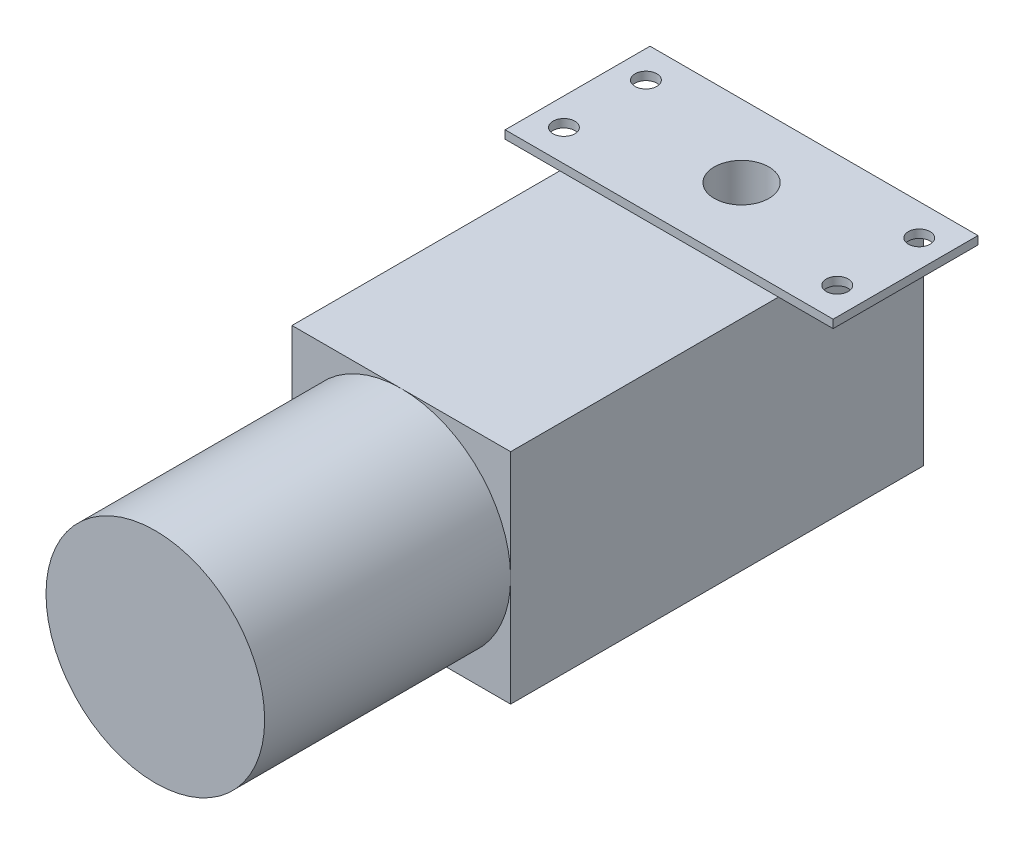
from build123d import *

# Parameters (mm, degrees)
SKETCH_1_W          = 80
SKETCH_1_H          = 80
EXTRUDE_1_DEPTH     = 241
SKETCH_2_W          = 120
SKETCH_2_H          = 53
EXTRUDE_2_DEPTH     = 3
SKETCH_3_R          = 4
CUT_EXTRUDE_1_DEPTH = 262.858740545
SKETCH_4_R          = 10
CUT_EXTRUDE_2_DEPTH = 262.858740545
SKETCH_5_OUTSIDE_W  = 178.346
SKETCH_5_OUTSIDE_H  = 141.346
SKETCH_5_OUTSIDE_R  = 40
CUT_EXTRUDE_3_DEPTH = 90


with BuildPart() as part:
    # 草图1 → 凸台-拉伸1 (new body)
    with BuildSketch(Plane.XY):
        Rectangle(SKETCH_1_W, SKETCH_1_H)
    extrude(amount=EXTRUDE_1_DEPTH)

    # 草图2 → 凸台-拉伸2 (add)
    with BuildSketch(Plane(origin=(0, 40, 0), x_dir=(1, 0, 0), z_dir=(0, 1, 0))):
        with Locations((0, -26.5)):
            Rectangle(SKETCH_2_W, SKETCH_2_H)
    extrude(amount=EXTRUDE_2_DEPTH)

    # 草图3 → 切除-拉伸1 (cut, through all)
    with BuildSketch(Plane(origin=(0, 43, 0), x_dir=(1, 0, 0), z_dir=(0, 1, 0))):
        with Locations(Location((-50, -11.5, 0), (0, 0, 180))):
            Circle(SKETCH_3_R)
        with Locations(Location((50, -11.5, 0), (0, 0, 180))):
            Circle(SKETCH_3_R)
        with Locations(Location((50, -41.5, 0), (0, 0, 180))):
            Circle(SKETCH_3_R)
        with Locations(Location((-50, -41.5, 0), (0, 0, 180))):
            Circle(SKETCH_3_R)
    extrude(amount=-CUT_EXTRUDE_1_DEPTH, mode=Mode.SUBTRACT)

    # 草图4 → 切除-拉伸2 (cut, through all)
    with BuildSketch(Plane(origin=(0, 43, 0), x_dir=(1, 0, 0), z_dir=(0, 1, 0))):
        with Locations(Location((0, -26.5, 0), (0, 0, 180))):
            Circle(SKETCH_4_R)
    extrude(amount=-CUT_EXTRUDE_2_DEPTH, mode=Mode.SUBTRACT)

    # 草图5 outside → 切除-拉伸3 (cut)
    with BuildSketch(Plane.XY.offset(241)):
        with Locations((0, 1.5)):
            Rectangle(SKETCH_5_OUTSIDE_W, SKETCH_5_OUTSIDE_H)
        with Locations(Location((0, 0, 0), (0, 0, 180))):
            Circle(SKETCH_5_OUTSIDE_R, mode=Mode.SUBTRACT)
    extrude(amount=-CUT_EXTRUDE_3_DEPTH, mode=Mode.SUBTRACT)


solid = part.part
